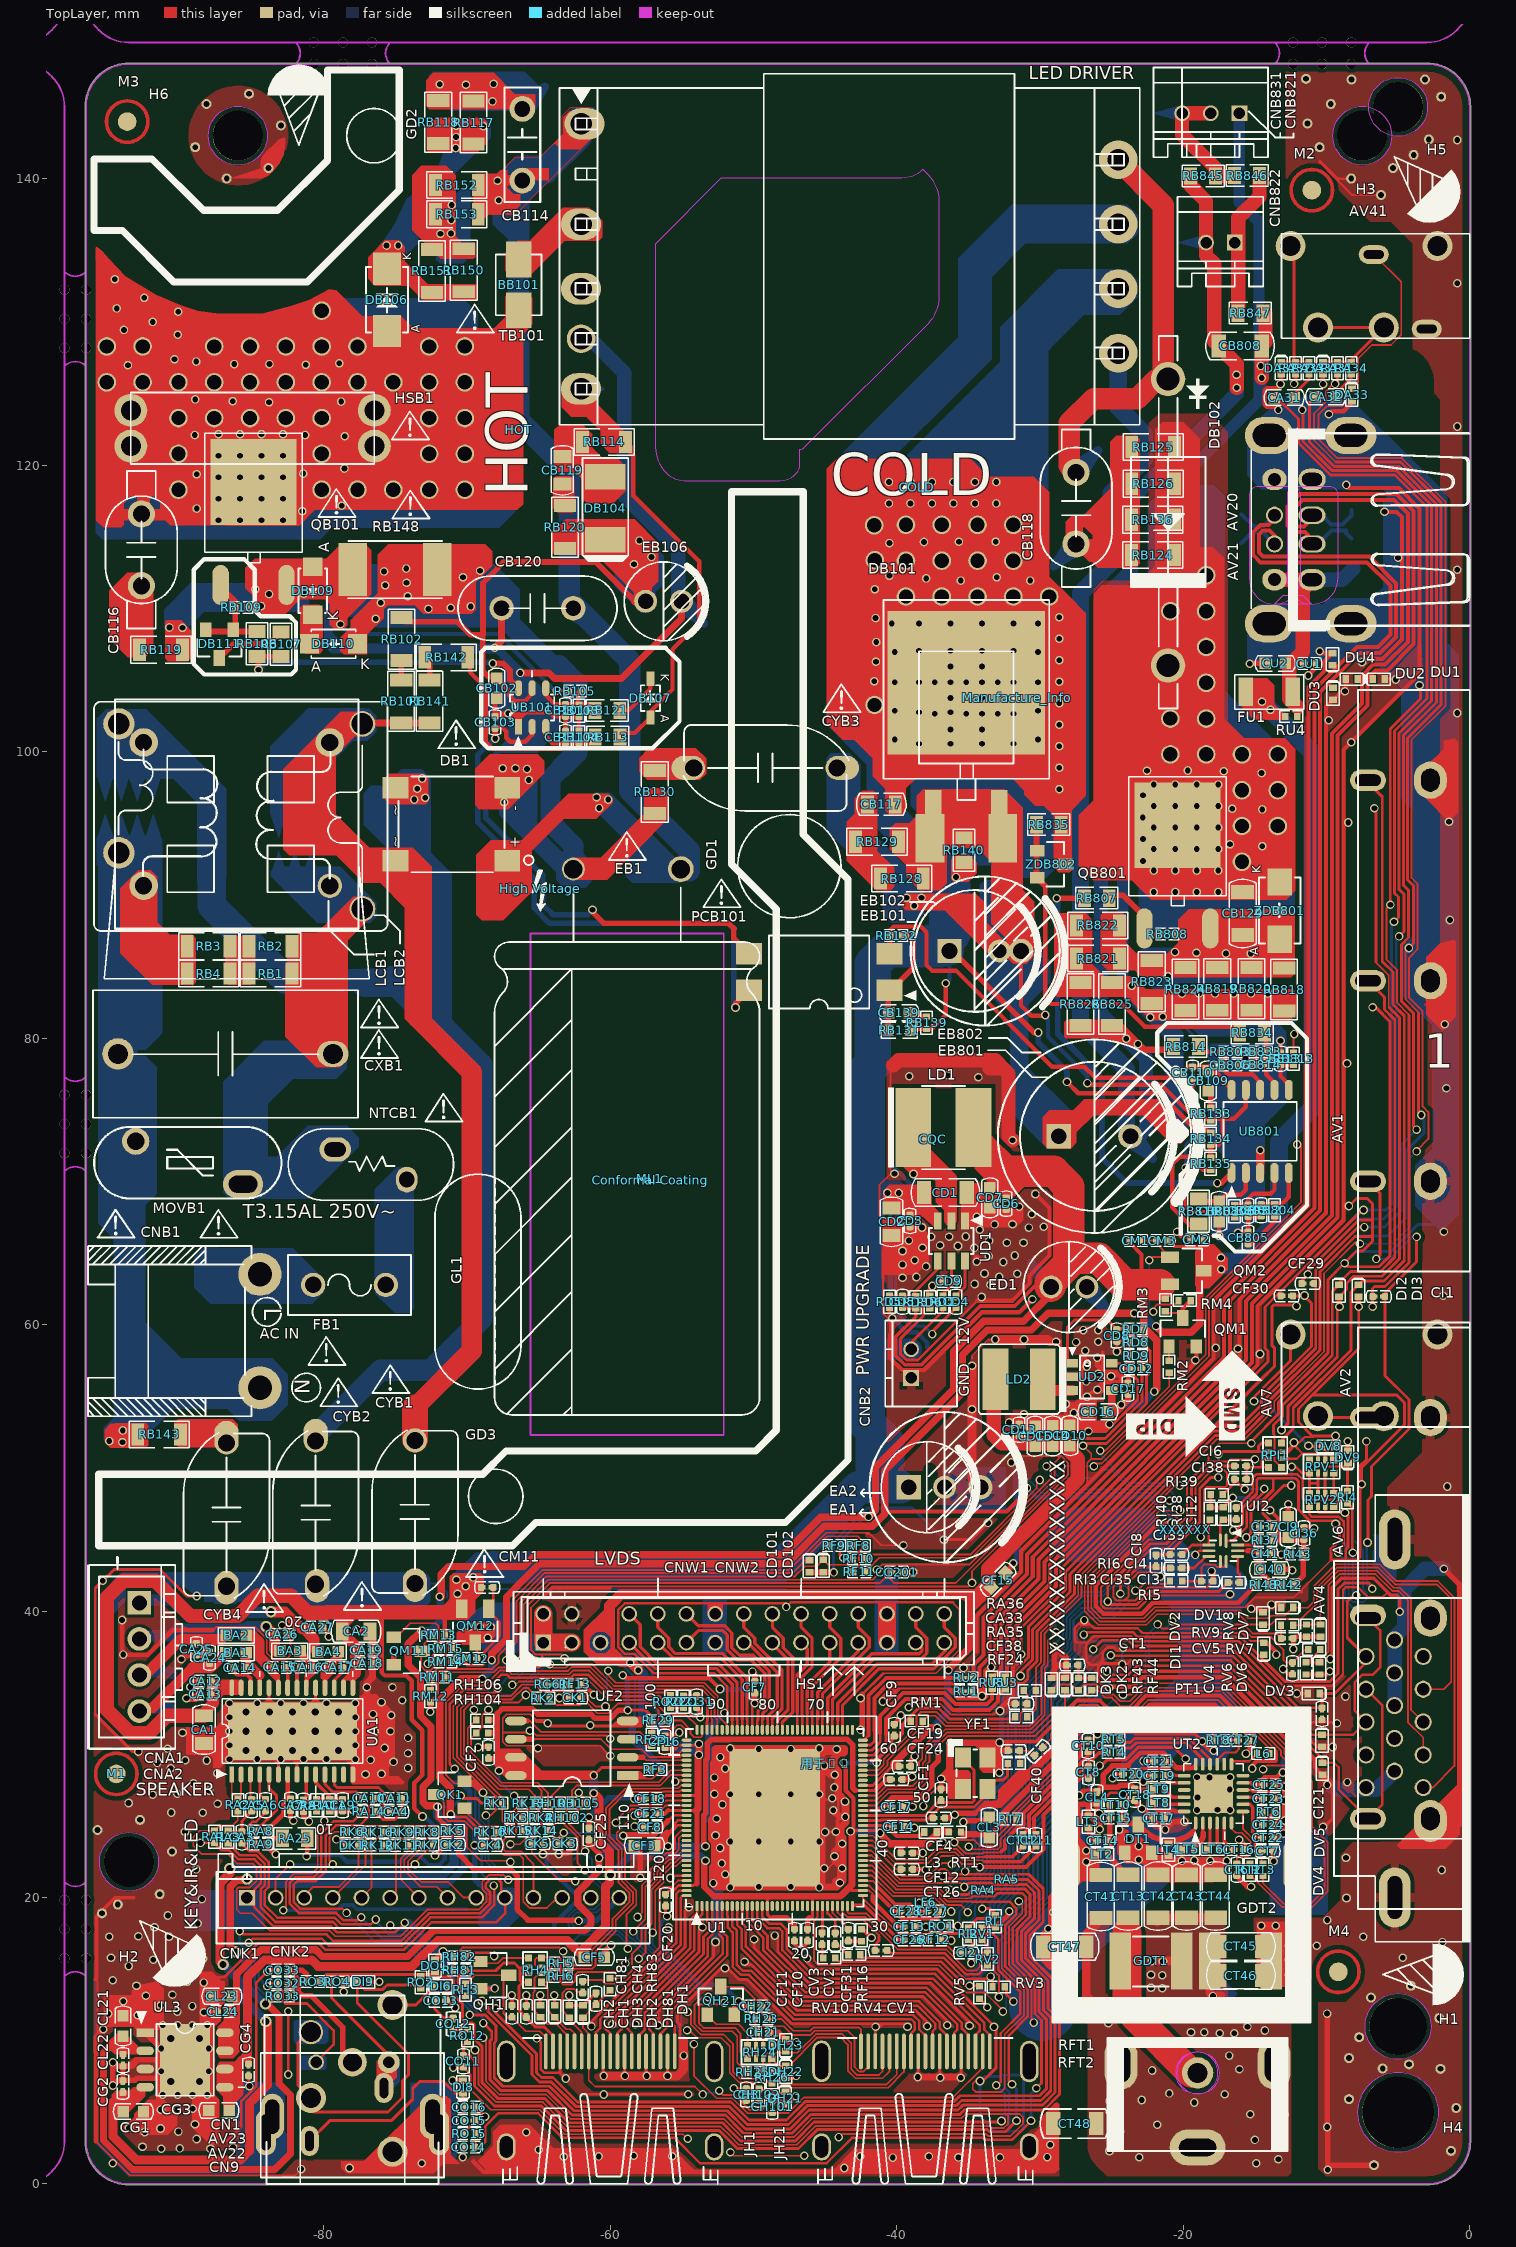
[diagram p0: TopLayer view]
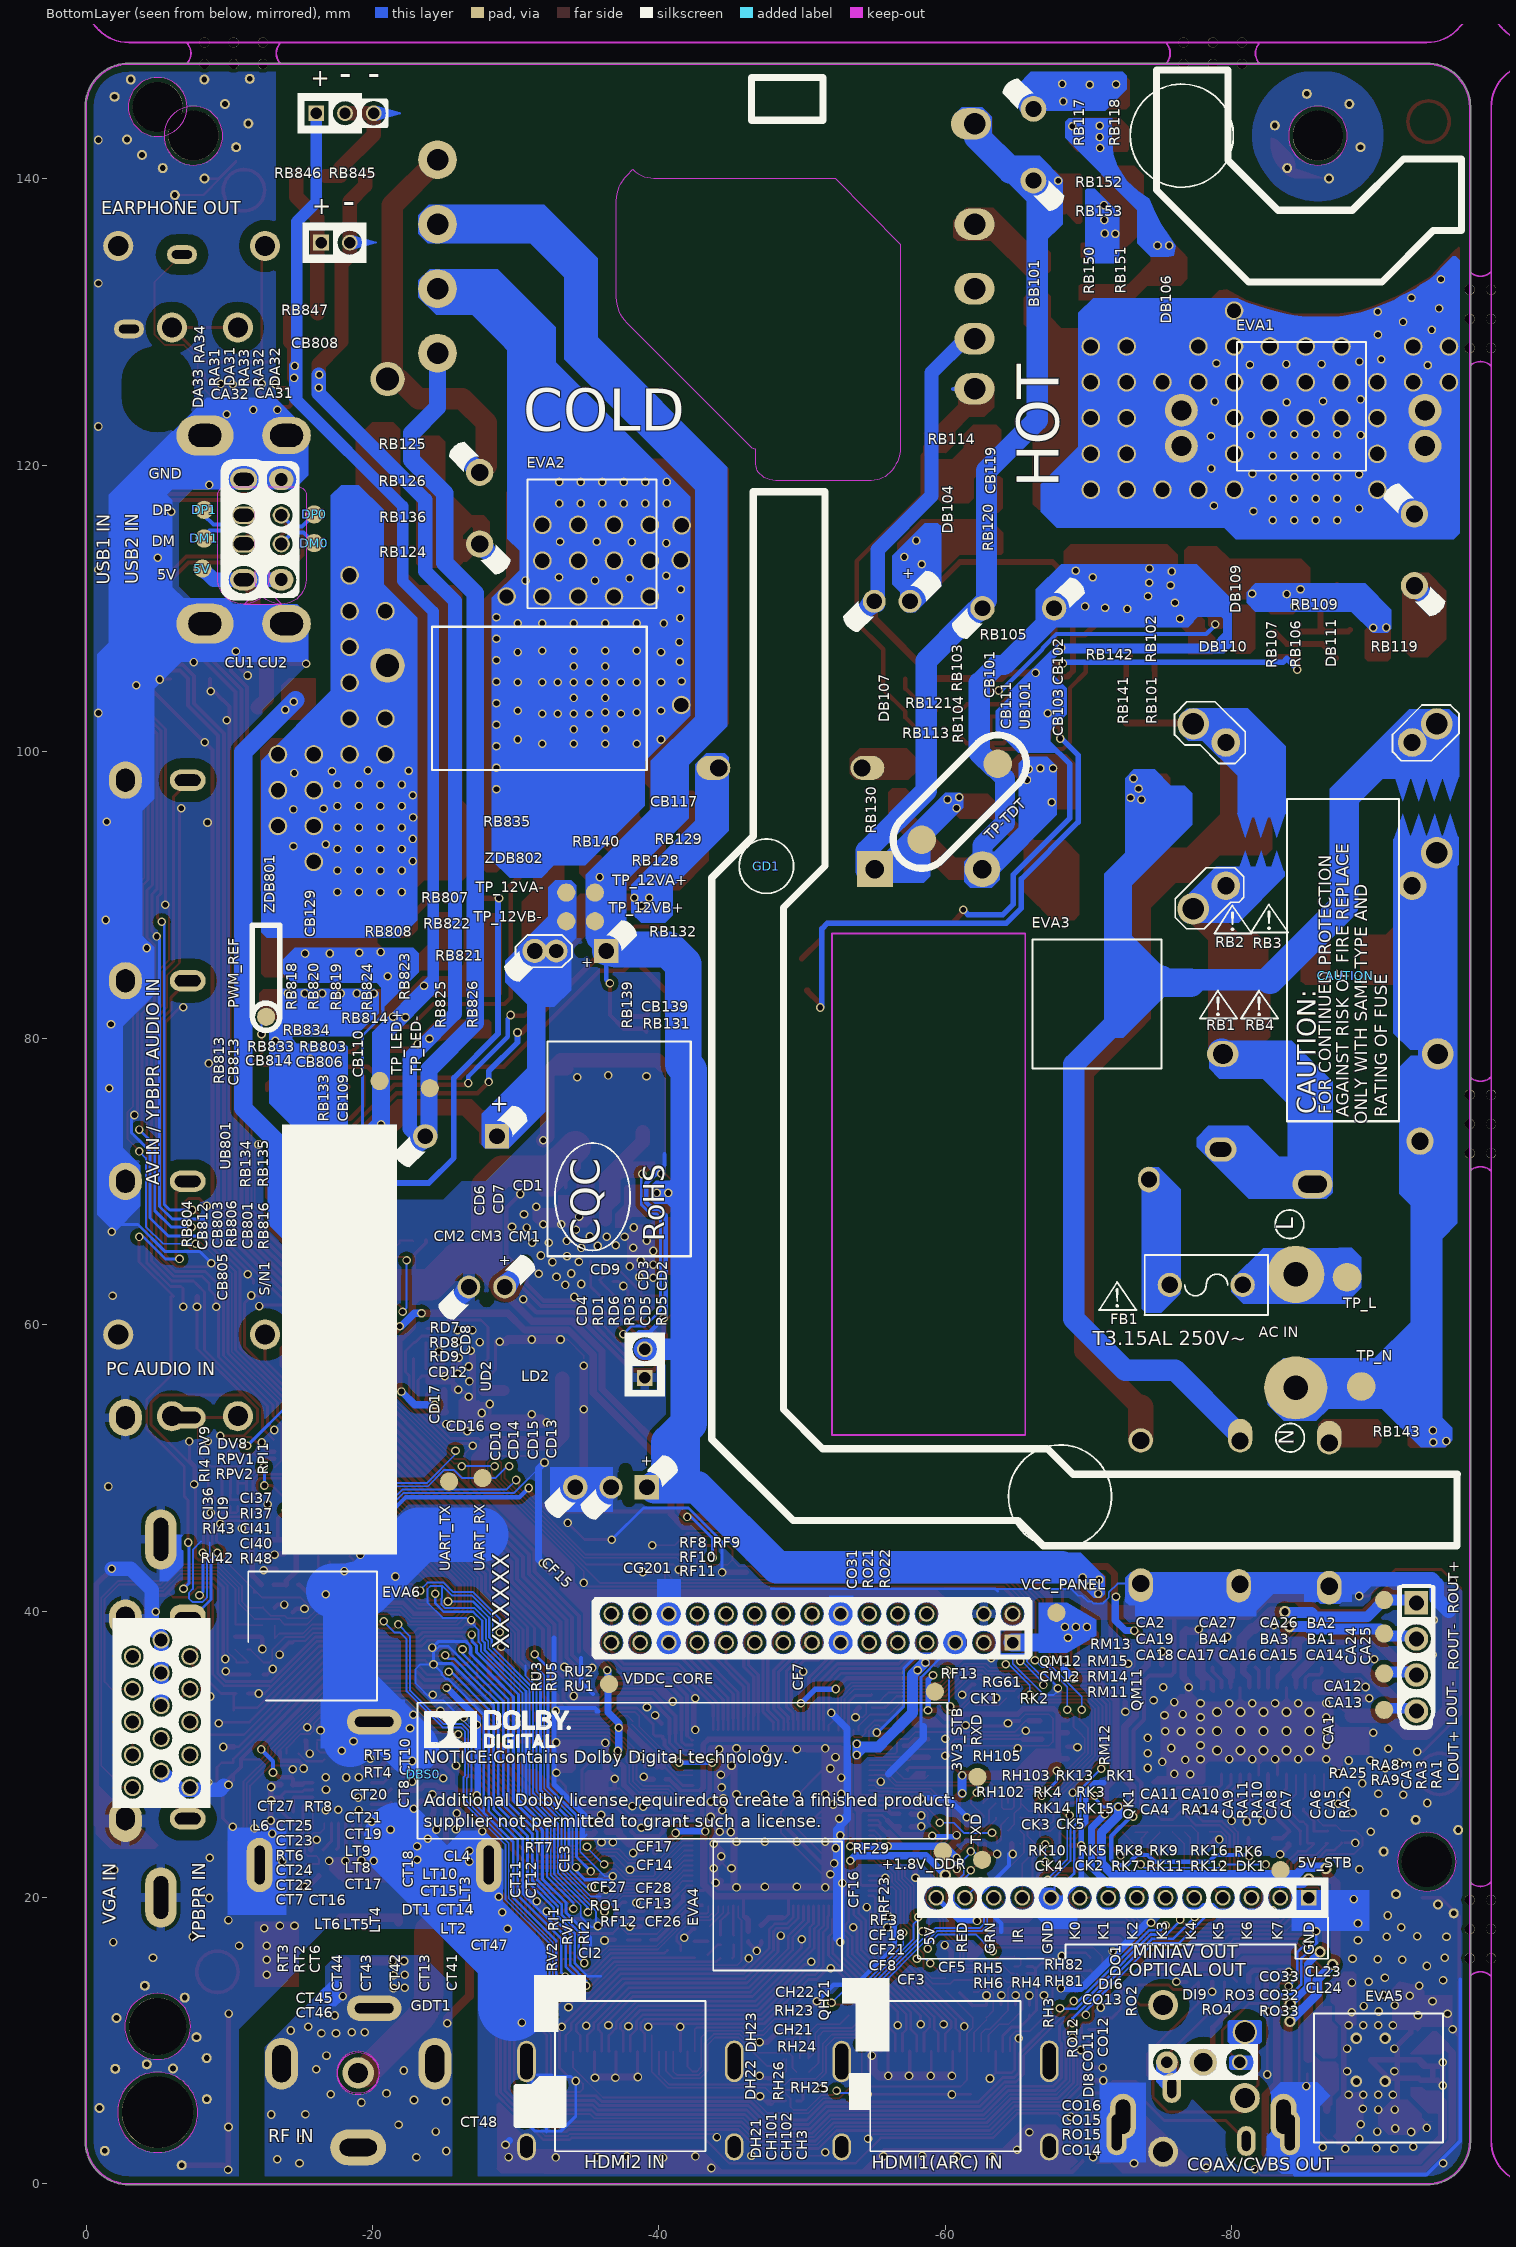
[diagram p1: BottomLayer view, seen from below]
# Altium PCB MISC86372.PcbDoc (part 1 of 16)
Units mm, origin at the board's own origin, x right, y up, seen from the top; angles counter-clockwise.
Board outline 96.73 x 148.13 mm, 2 copper layers (TopLayer, BottomLayer), stack 1.571 mm thick; 578 components, 318 nets, 2702 pads, 836 vias.

## Layer stack, top to bottom
TopLayer: signal copper 0.0356
Dielectric: core 1.5, FR-4, Dk 4.8
BottomLayer: signal copper 0.0356

## Board outline
-96.664,3 -96.664,76.338 -96.664,76.25 ccw(c-96.6,76.25) -96.664,76.249 -96.664,76.25 -96.664,145 cw(c-93.6,145) -93.6,148.064 -3,148.064 cw(c-3,145) 0.064,145 0.064,3 cw(c-3,3) -3,-0.064 -93.6,-0.064 cw(c-93.6,3)

## Design rules (kind name [scope] priority, off if disabled: settings)
Clearance ■KEEPOUT_18mil [(IsTrack Or IsArc) And (AsMM(Width) < 1) And IsKeepOut vs Not IsPad] p1: gap=0.457
Clearance ■HOT_7.2mm [InNetClass('HOT') vs InNetClass('All Nets') And (Not InNetClass('HOT'))] p2: gap=8
Clearance ■DFM_NPTH_10mil [(IsPadHoleValid And (PadIsPlated=false) Or IsPad And ((AsMM(PadXSize_AllLayers) < 1) or (AsMM(PadYSize_AllLayers) < 1 )) And IsKeepout) OR HasFootprintPad('ASSE*','0') vs Not IsPad] p3: gap=0.254
Clearance ■DFM_20mil [(IsTrack or IsArc or IsPad) And IsKeepOut vs IsTrack or IsArc or InPoly] p4: gap=0.508
Clearance ■C_RJ45_2mm [InNetClass('RJ45') vs Not InNetClass('RJ45') AND InNet('*')] p5: gap=2
Clearance ■PWR_A12_8mil [((InNetClass('PWR_A12_8mil') or InNet('*12V*') or InNet('*24V*') or InNet('*PVCC*') or InNet('*19V*') or InNet('*AMP*POWER*') or InNet('*AMP*VCC*') or InNet('*LNB*')) And Not InNetClass('A12_8mil_EXC')) and Not IsPad vs Not InPoly] p6: gap=0.203
Clearance ■PS_L2All_3.2mm [InNet('L-1') vs InNet('*')] p7: gap=3.2
Clearance ■PS_L2LN_1.5mm [InNet('L') Or InNet('L-2') Or InNet('L-3') Or InNet('L-4') Or InNet('L-5') Or InNet('L-6') vs InNet('L-N') And Not(InNet('L') Or InNet('L-2') Or InNet('L-3') Or InNet('L-4') Or InNet('L-5') Or InNet('L-6'))] p8: gap=1.5
Clearance ■PS_N2LN_1.5mm [InNet('N') OR InNet('N-1') OR InNet('N-2') OR InNet('N-3') OR InNet('N-4') OR InNet('N-5') OR InNet('N-6') vs InNet('L-N') And Not (InNet('N') OR InNet('N-1') OR InNet('N-2') OR InNet('N-3') OR InNet('N-4') OR InNet('N-5') OR InNet('N-6'))] p9: gap=1.5
Clearance ■PS_L2LN_3mm [InNet('L') Or InNet('L-2') Or InNet('L-3') Or InNet('L-4') Or InNet('L-5') Or InNet('L-6') vs InNet('*') And Not (InNet('L-N') Or InNet('L') Or InNet('L-2') Or InNet('L-3') Or InNet('L-4') Or InNet('L-5') Or InNet('L-6') Or OnLayer('KeepOutLayer'))] p10: gap=3
Clearance ■PS_N2LN_3mm [InNet('N') OR InNet('N-1') OR InNet('N-2') OR InNet('N-3') OR InNet('N-4') OR InNet('N-5') OR InNet('N-6') vs InNet('*') And Not (InNet('L-N') Or InNet('N') OR InNet('N-1') OR InNet('N-2') OR InNet('N-3') OR InNet('N-4') OR InNet('N-5') OR InNet('N-6') Or OnLayer('KeepOutLayer'))] p11: gap=3
Clearance ■SIP2GND_8mil [HasFootprint('SIP*') vs InPoly] p12: gap=0.203
Clearance ■C_BGA_0P65 [HasFootprint('BGA*0.65*') vs InPoly] p13: gap=0.127
Clearance ■C_BGA_0P8 [HasFootprint('BGA*0.8*') vs InPoly] p14: gap=0.14
Clearance ■Poly_4mil [InPolygonClass('Poly_4mil') vs Not InPoly] p15: gap=0.102
Clearance ■Poly_5mil [InPolygonClass('Poly_5mil') vs Not InPoly] p16: gap=0.127
Clearance ■Poly_6.2mil [InPolygonClass('Poly_6.2mil') vs Not InPoly] p17: gap=0.157
Clearance ■Poly_8mil [InPolygonClass('Poly_8mil') vs Not InPoly] p18: gap=0.203
Clearance ■C_RFGND_1.8mm [InNet('RFGND') vs Not (InNet('RF*IN*') OR InNet('NetCT28*'))] p19: gap=1.8
Clearance ■ESD_10mil [HasFootprint('*IEC*') Or HasFootprint('*-F1*') Or HasFootprint('ANT-RF*')] p20: gap=0.254
Clearance ■ESD_20mil [HasFootprint('*SHIELD*')] p21: gap=0.508
Clearance ■GND_12mil [InNet('GND') vs InPoly] p22: gap=0.305
Clearance ■ESD_30mil [(HasFootprint('SCART*') OR HasFootprint('AV*') OR HasFootprint('DB15*') OR HasFootprint('PHONE*')) vs OnBottomLayer] p23: gap=0.762
Clearance ■ESD_NT_30mil [HasFootprint('SCART*') Or HasFootprint('PHONE-HD-12') Or HasFootprint('PHONE-HD-17') Or HasFootprint('PHONE-HD-10') Or HasFootprint('PHONE-HD-26') vs InNet('GND') And OnTopLayer] p24: gap=0.762
Clearance ■DFM_TH_5mil [HasFootprint('GND') or HasFootprint('TP*') or HasFootprint('MARK*') or HasFootprint('SPARK_GAP') or HasFootprint('USB-HD-3-2') or HasFootprint('PHONE-HS-20') and Not IsRegion vs OnBottomlayer And IsPad OR IsPadHoleValid] p25: gap=0.127
Clearance ■DFM_HS60_5mil [InPadClass('HS60') vs InPadClass('HS60') OR IsPadHoleValid and not InPadClass('VIA5')] p26: gap=0.127
Clearance ■DFM_BCR_4mm [IsPadHoleValid vs IsBoardCutoutRegion] p27: gap=4
Clearance ■DFM_TH_4mm [OnBottomlayer And IsSMTPin vs IsPadHoleValid and not InPadClass('VIA5')] p28: gap=4
Clearance ■DFM_HS60_4mm [InPadClass('HS60') vs IsPad and OnBottomlayer] p29: gap=4
Clearance ■VIA2VIA_6.2mil [(IsVia OR InPadClass('VIA5')) And Not (IsVia And (AsMM(HoleDiameter) = 0.1)) vs (IsVia OR InPadClass('VIA5')) And Not (IsVia And (AsMM(HoleDiameter) = 0.1))] p30: gap=0.157
Clearance ■VIA2VIA_16.2mil [(IsVia OR InPadClass('VIA5')) And Not (IsVia And (AsMM(HoleDiameter) = 0.1)) vs (IsVia OR InPadClass('VIA5')) And Not (IsVia And (AsMM(HoleDiameter) = 0.1))] p31: gap=0.411
Clearance ■VIA2PAD_BGA_5mil [HasFootprint('BGA*') and IsPad vs (IsVia OR InPadClass('VIA5')) And Not (IsVia And (AsMM(HoleDiameter) = 0.1))] p32: gap=0.127
Clearance ■VIA2PAD_6mil [IsVia And Not (IsVia And (AsMM(HoleDiameter) = 0.1)) vs ISPAD and Not HasFootprintPad('*','EPAD') and Not HasFootprintPad('*','257') and Not HasFootprintPad('TP','*') and Not HasFootprintPad('GND','JP*') and Not HasFootprintPad('LQFP216/0.4-2','217') and Not HasFootprintPad('QFP16*','17') and Not HasFootprintPad('QFN16*','17') and Not HasFootprintPad('QFN20*','21') and Not HasFootprintPad('QFN24*','25') and Not HasFootprintPad( 'QFN24*','29') and Not HasFootprintPad('QFN28*','29') and Not HasFootprintPad('QFN32*','33') and Not HasFootprintPad('QFN36*','37') and Not HasFootprintPad('QFN36*','0') and Not HasFootprintPad('QFN32*','0') and Not HasFootprintPad('QFN40*','41') and Not HasFootprintPad('QFN48*','49') and Not HasFootprintPad('LQFP48/0.5-2','49') and Not HasFootprintPad('*SSOP32*','33') and Not HasFootprintPad('SOP8*','9') and Not HasFootprintPad('WSON8/1.27*','9') and Not HasFootprintPad('DFN10/0.5-1*','11') and Not HasFootprintPad('SON16/0.4','9') and Not HasFootprintPad('MSOP10/0.5-1','11') and Not HasFootprintPad('QFN56/0.5','57') and Not HasFootprintPad('LGA31/0.5','3*') and Not InPadClass('VIA_HS60') and Not HasFootprintPad('TSSOP16/0.65-3','17') and Not HasFootprintPad('QFP128/0.5-2','129') and Not HasFootprintPad('QFP128/0.4-5','129') and Not HasFootprintPad('PQFP48*','49') and Not HasFootprintPad('QFP156/0.4-1','157') and Not HasFootprintPad('D2PAK3-TO-252','2') and Not HasFootprintPad('D2PAK3','2')] p33: gap=0.152
Clearance ■PAD2VIA5_6mil [IsPad And ((AsMM(PadXSize_AllLayers) < 2.5) or ((AsMM(PadYSize_AllLayers) < 2.5))) And Not InPadclass('HS60') vs InPadClass('VIA5')] p34: gap=0.152
Clearance "■12mil for Polygon" [InPoly] p35: gap=0.305
Clearance 8mil [All] p36 off: gap=0.203
Clearance 7mil [All] p37 off: gap=0.178
Clearance 6.2mil [All] p38 off: gap=0.157
Clearance 6mil [All] p39 off: gap=0.152
Clearance 5.8mil [All] p40 off: gap=0.147
Clearance 5mil [Not ((IsTrack Or IsArc) And (Layer = 'KeepOutLayer')) vs Not (IsPad or ((IsTrack Or IsArc) And (Layer = 'KeepOutLayer')))] p41 off: gap=0.127
Clearance 4.5mil [Not ((IsTrack Or IsArc) And (Layer = 'KeepOutLayer')) vs Not (IsPad or ((IsTrack Or IsArc) And (Layer = 'KeepOutLayer')))] p42 off: gap=0.114
Clearance "4mil for Minimum" [Not ((IsTrack Or IsArc) And (Layer = 'KeepOutLayer')) vs Not (IsPad or ((IsTrack Or IsArc) And (Layer = 'KeepOutLayer')))] p43: gap=0.102
ComponentClearance ■DFMC_1mm [Not (InComponentClass('Co-Layout') Or HasFootprint('GND')) And (HasFootprint('T/E*') Or HasFootprint('T/PQ*') Or HasFootprint('USB*') Or HasFootprint('HDMI*') Or HasFootprint('USB*') Or HasFootprint('DC-*') Or HasFootprint('AV*') Or HasFootprint('ANT*') Or HasFootprint('PHONE*') Or HasFootprint('CICARD*') Or HasFootprint('CARD*') Or HasFootprint('DVI*') Or HasFootprint('DB*') Or HasFootprint('DP*') Or HasFootprint('DISPLAYPORT*') Or HasFootprint('OPTICAL*') Or HasFootprint('SCART*') Or HasFootprint('RJ45*') Or HasFootprint('USB*') Or HasFootprint('T-*') Or HasFootprint('T/*') Or HasFootprint('200-*') Or HasFootprint('ZhiJia*') Or HasFootprint('Dianpian*') Or HasFootprint('TanPian*') Or HasFootprint('P(*')) vs Not (InComponentClass('Co-Layout') Or HasFootprint('GND'))] p1 off: gap=1 collisioncheckmode=3 verticalgap=1 showdistances=FALSE
ComponentClearance ■DFMC_0.5mm [Not (InComponentClass('Co-Layout') Or HasFootprint('SO-23') Or HasFootprint('DIODE-s0402') Or HasFootprint('GND')) And (HasFootprint('M-*') Or HasFootprint('BGA*') Or HasFootprint('QFP*') Or HasFootprint('QFN*') Or HasFootprint('*DFN*') Or HasFootprint('*SOP*') Or HasFootprint('LGA*') Or HasFootprint('SOIC*') Or HasFootprint('EC*') Or HasFootprint('AC-*') Or HasFootprint('DIODE*') Or HasFootprint('XTAL*') Or HasFootprint('SO-*') Or HasFootprint('L/LC*') Or HasFootprint('L(*') Or HasFootprint('WIFI*') Or HasFootprint('SATA*') Or HasFootprint('POGO*') Or HasFootprint('SOT-223') Or HasFootprint('TO-252') Or HasFootprint('TO-263') Or HasFootprint('KEY*') Or HasFootprint('SW*') Or HasFootprint('DIP*') Or HasFootprint('SIP*') Or HasFootprint('DIP*') Or HasFootprint('CON*') Or HasFootprint('FFC*') Or HasFootprint('FPC*') Or HasFootprint('GDT*') Or HasFootprint('R2512*') Or HasFootprint('R2725*') Or HasFootprint('L2012*') Or HasFootprint('L2520*')) vs Not (InComponentClass('Co-Layout') Or HasFootprint('SO-23') Or HasFootprint('DIODE-s0402') Or HasFootprint('GND'))] p2 off: gap=0.5 collisioncheckmode=3 verticalgap=0.5 showdistances=FALSE
ComponentClearance ■DFMC_0.4mm [Not (InComponentClass('Co-Layout') Or HasFootprint('GND')) And (HasFootprint('C0201*') Or HasFootprint('C0402*') Or HasFootprint('C0603*') Or HasFootprint('C0805*') Or HasFootprint('C1206*') Or HasFootprint('C1210*') Or HasFootprint('R0201*') Or HasFootprint('R0402*') Or HasFootprint('R0603*') Or HasFootprint('R0805*') Or HasFootprint('R*0402*') Or HasFootprint('L0201*') Or HasFootprint('L0402*') Or HasFootprint('L0603*') Or HasFootprint('L0805*') Or HasFootprint('L1206*') Or HasFootprint('DIODE-s0402')) vs Not (InComponentClass('Co-Layout') Or HasFootprint('GND')) And (HasFootprint('C0201*') Or HasFootprint('C0402*') Or HasFootprint('C0603*') Or HasFootprint('C0805*') Or HasFootprint('C1206*') Or HasFootprint('C1210*') Or HasFootprint('R0201*') Or HasFootprint('R0402*') Or HasFootprint('R0603*') Or HasFootprint('R0805*') Or HasFootprint('R*0402*') Or HasFootprint('L0201*') Or HasFootprint('L0402*') Or HasFootprint('L0603*') Or HasFootprint('L0805*') Or HasFootprint('L1206*') Or HasFootprint('DIODE-s0402'))] p3 off: gap=0.4 collisioncheckmode=3 verticalgap=0.4 showdistances=FALSE
ComponentClearance ■DFMC_0.36mm [Not (InComponentClass('Co-Layout') Or HasFootprint('GND')) And HasFootprint('R1206*') vs Not (InComponentClass('Co-Layout') Or HasFootprint('GND')) And HasFootprint('R1206*')] p4 off: gap=0.36 collisioncheckmode=3 verticalgap=0.36 showdistances=FALSE
ComponentClearance ■DFMC_0.25mm [Not (InComponentClass('Co-Layout') Or HasFootprint('GND')) vs Not (InComponentClass('Co-Layout') Or HasFootprint('GND'))] p5 off: gap=0.25 collisioncheckmode=3 verticalgap=0.25 showdistances=FALSE
DiffPairsRouting ■DiffPair_USB_DiffPairsRouting [InDifferentialPairClass('USB')] p1: maxlimit=0.127 minlimit=0.102 mostfreqgap=0.127 maxuncoupledlength=5.08
DiffPairsRouting ■DiffPair_LVDS_DiffPairsRouting [InDifferentialPairClass('LVDS')] p2: maxlimit=0.127 minlimit=0.102 mostfreqgap=0.127 maxuncoupledlength=12.7
DiffPairsRouting ■DiffPair_HDMI_DiffPairsRouting [InDifferentialPairClass('HDMI')] p3: maxlimit=0.127 minlimit=0.102 mostfreqgap=0.127 maxuncoupledlength=5.08
DiffPairsRouting [All] p4: maxlimit=0.254 minlimit=0.254 mostfreqgap=0.254 maxuncoupledlength=12.7
FabricationTestPointUsage TestPointUsage [All] p1: valid=0 allowmultiple=FALSE
FabricationTestpoint Testpoint [All] p1: side=3 testpointundercomponent=TRUE minsize=1.016 maxsize=2.54 preferedsize=1.524 minholesize=0.508 maxholesize=1.016 preferedholesize=0.813 testpointgrid=0.025 allowsidetop=TRUE allowsidebottom=TRUE usegrid=TRUE gridtolerance=0
HoleSize HoleSize_VIA [ISVIA] p1 off: absolutevalues=TRUE maxlimit=0.6 minlimit=0.2 maxpercent=80.000 minpercent=20.000
HoleToHoleClearance Hole2Hole [All] p1 off: gap=0.457 allowstackedmicrovias=FALSE
MatchedLengths DiffPair_USB_MatchedLengths [InDifferentialPairClass('USB')] p1: tolerance=2.54 checknetsindiffpair=TRUE checkdiffpairvsdiffpair=FALSE checkothers=FALSE
MatchedLengths DiffPair_LVDS_MatchedLengths [InDifferentialPairClass('LVDS')] p2: tolerance=2.54 checknetsindiffpair=TRUE checkdiffpairvsdiffpair=FALSE checkothers=FALSE
MatchedLengths DiffPair_HDMI_MatchedLengths [InDifferentialPairClass('HDMI')] p3: tolerance=2.54 checknetsindiffpair=TRUE checkdiffpairvsdiffpair=FALSE checkothers=FALSE
MinimumAnnularRing [All] p1: minimumring=0.1
MinimumSolderMaskSliver ■MiniSolderMaskSliver [All] p1 off: minsoldermaskwidth=0.098
NetAntennae [Not (HasFootprint('ANT-7') or HasFootprint('ANT-BLUECORE'))] p1: netantennaetolerance=1.016
PermittedLayers [All] p1: toplayerpermitted=TRUE bottomlayerpermitted=TRUE
PlaneClearance ■Plane_ESD_30mil [(HasFootprint('SCART*') OR HasFootprint('AV*') OR HasFootprint('DB15*') OR HasFootprint('PHONE*'))] p1: clearance=0.762
PlaneClearance ■Plane_All_9mil [All] p2: clearance=0.229
PlaneConnect ■PlaneOverAll [IsVia or InPadClass('VIA5') Or HasFootprint('ASSE*') OR InPadclass('HS60')] p1: planeconnectstyle=Direct reliefexpansion=0.508 reliefentries=4 reliefconductorwidth=0.254 reliefairgap=0.254
PlaneConnect ■PlaneConnect [All] p2: planeconnectstyle=Relief reliefexpansion=0.305 reliefentries=4 reliefconductorwidth=0.762 reliefairgap=0.305
PolygonConnect ■PourOverAll [IsVia Or InPadclass('HS60') Or InPadClass('VIA5') Or HasFootprint('ASSE*') Or HasFootprint('DIODE-S0402') Or HasFootprint('RCL0524P') Or HasFootprint('SOT-89') OR HasFootprint('SOT-223') OR HasFootprint('TO-252') OR HasFootprint('TO-263') OR HasFootprint('DIODE') OR HasFootprint('SW-HS-2') OR HasFootprint('HDMI*') OR HasFootprint('SO-8B') OR HasFootprint('GND') OR HasFootprint('PHONE*') OR HasFootprint('DIP18/2.54-2') OR HasFootprint('DIP18/2.54-1') OR HasFootprint('UFL-R-SMT-1') OR HasFootprint('WIFI') OR HasFootprint('UM02BS') OR HasFootprint('*SCART*') OR HasFootprint('TSOT23-8/0.65') OR HasFootprint('*SOT-23-*') OR HasFootprint('SOP23-5-1') OR HasFootprint('SOP6/0.95') OR HasFootprint('M-WIFI-2-M603USA1') OR HasFootprint('M-MT7632U') OR HasFootprint('SOP8/1.27') OR HasFootprint('SOP8/1.27-3') vs IsPolygon] p1: connectstyle=Direct reliefconductorwidth=0.254 reliefentries=4 polygonreliefangle="90 Angle"
PolygonConnect ■BGA_0P65 [HasFootprint('BGA*0.65*') vs IsPoly] p2: connectstyle=Relief reliefconductorwidth=0.203 reliefentries=4 polygonreliefangle="45 Angle"
PolygonConnect ■BGA_0P8 [HasFootprint('BGA*0.8*') vs IsPoly] p3: connectstyle=Relief reliefconductorwidth=0.229 reliefentries=4 polygonreliefangle="45 Angle"
PolygonConnect ■Polygon_RFGND [InNet('RFGND')] p4: connectstyle=Direct reliefconductorwidth=0.254 reliefentries=4 polygonreliefangle="90 Angle"
PolygonConnect ■ESD_SCART [HasFootprint('SCART*') vs IsPolygon And onBottomlayer] p5: connectstyle=Direct reliefconductorwidth=0.762 reliefentries=4 polygonreliefangle="90 Angle"
PolygonConnect ■C2Polygon_35mil [HasFootprint('EC*') vs IsPolygon] p6: connectstyle=Relief reliefconductorwidth=0.889 reliefentries=4 polygonreliefangle="90 Angle"
PolygonConnect ■C2Polygon_30mil [(HasFootprint('*0805*') OR HasFootprint('*1206*')) vs IsPolygon] p7: connectstyle=Relief reliefconductorwidth=0.762 reliefentries=4 polygonreliefangle="90 Angle"
PolygonConnect ■C2Polygon_25mil [HasFootprint('*0603*') Or IsThruPin vs IsPolygon] p8: connectstyle=Relief reliefconductorwidth=0.635 reliefentries=4 polygonreliefangle="90 Angle"
PolygonConnect ■C2Polygon_12mil [IsSMTPin vs IsPolygon] p9: connectstyle=Relief reliefconductorwidth=0.305 reliefentries=4 polygonreliefangle="90 Angle"
RoutingVias 0.6_0.4 [All] p1: holewidth=0.4 width=0.6 viastyle="Through Hole" minholewidth=0.4 minwidth=0.6 maxholewidth=0.4 maxwidth=0.6
RoutingVias 0.8_0.5 [All] p2 off: holewidth=0.5 width=0.8 viastyle="Through Hole" minholewidth=0.5 minwidth=0.8 maxholewidth=0.5 maxwidth=0.8
RoutingVias 0.5_0.3 [All] p3 off: holewidth=0.3 width=0.5 viastyle="Through Hole" minholewidth=0.3 minwidth=0.5 maxholewidth=0.3 maxwidth=0.5
RoutingVias 0.45_0.25 [All] p4 off: holewidth=0.25 width=0.45 viastyle="Through Hole" minholewidth=0.25 minwidth=0.45 maxholewidth=0.25 maxwidth=0.45
RoutingVias 0.4_0.2 [All] p5 off: holewidth=0.2 width=0.4 viastyle="Through Hole" minholewidth=0.2 minwidth=0.4 maxholewidth=0.2 maxwidth=0.4
RoutingVias 0.25_0.1 [All] p6 off: holewidth=0.1 width=0.25 viastyle="Through Hole" minholewidth=0.1 minwidth=0.25 maxholewidth=0.1 maxwidth=0.25
SMDNeckDown ■SMDNeckDown_Chip [HasFootprint('FFC*') or HasFootprint('QFP*') or HasFootprint('QFN*') or HasFootprint('HDMI*') or HasFootprint('BGA*')] p1: percent=100.000
SMDToCorner [All] p1 off: distance=40000
ShortCircuit ■ShortCircuit_ViaOnEpad [HasFootprintPad( '*','EPAD') vs IsVia AND InNet('*')] p1: allowed=TRUE
ShortCircuit ■ShortCircuit_JP [HasFootprintPad( 'GND','JP_1K') vs HasFootprintPad( 'GND','JP_2K')] p2: allowed=TRUE
ShortCircuit ■ShortCircuit_0402 [HasFootprintPad('R0402SC','1') OR HasFootprintPad('R0402SC','2') vs HasFootprintPad('R0402SC','3')] p3: allowed=TRUE
ShortCircuit ■ShortCircuit_0603 [HasFootprintPad('R0603SC','1') OR HasFootprintPad('R0603SC','2') vs HasFootprintPad('R0603SC','3')] p4: allowed=TRUE
ShortCircuit ■ShortCircuit_0805 [HasFootprintPad('R0805SC','1') OR HasFootprintPad('R0805SC','2') vs HasFootprintPad('R0805SC','3')] p5: allowed=TRUE
ShortCircuit ■ShortCircuit_1206 [HasFootprintPad('R1206SC','1') OR HasFootprintPad('R1206SC','2') vs HasFootprintPad('R1206SC','3')] p6: allowed=TRUE
ShortCircuit ■ShortCircuit [InNet('*')] p7: allowed=FALSE
SilkToSilkClearance ■Silk2Silk [All] p1: silktosilkclearance=0.127
SilkscreenOverComponentPads ■SilkOverPads [IsText] p1: minsilkscreentomaskgap=0.003
SolderMaskExpansion ■SolderMask_VIA [IsVia] p1: expansion=0.13
SolderMaskExpansion ■SolderMask_All [All] p2: expansion=0.051
UnRoutedNet ■UnRoutedNet [All] p1:
ViasUnderSMD [All] p1: allowed=FALSE
Width ■Width_2.5mm [InFromToClass('Width_2.5mm')] p1: maxlimit=2.5 minlimit=2.5 preferedwidth=2.5
Width ■Width_1.5mm [InFromToClass('Width_1.5mm')] p2: maxlimit=1.5 minlimit=1.5 preferedwidth=1.5
Width ■DiffPair_USB_Width [InDifferentialPairClass('USB')] p3: maxlimit=0.279 minlimit=0.102 preferedwidth=0.279
Width ■DiffPair_LVDS_Width [InDifferentialPairClass('LVDS')] p4: maxlimit=0.178 minlimit=0.102 preferedwidth=0.178
Width ■DiffPair_HDMI_Width [InDifferentialPairClass('HDMI')] p5: maxlimit=0.178 minlimit=0.102 preferedwidth=0.178
Width [All] p6: maxlimit=12.7 minlimit=0.076 preferedwidth=0.203
14 further rules are at their usual default settings.

## Classes and differential pairs
net class POWER: 12V 12V_OVP BRO D_QB101 D_QB801 FB GND L L-1 L-2 L-3 L-N LED_FB N-1 N-2 N-3 NetBB101_2 NetCB101_1 NetCB102_1 NetCB103_1 NetCB109_2 NetCB114_2 NetCB116_2 NetCB117_2 NetCB118_2 NetCB119_1 NetCB119_2 NetCB139_1 NetCB139_2 NetCB801_1 NetCB803_1 NetCB805_2 NetCB806_1 NetCB812_2 NetCB813_2 NetCB814_1 NetCNB821_2 NetCNB822_1 NetCYB3_1 NetDB107_K NetDB109_A NetDB109_K NetDB111_1 NetDB111_2 NetQB801_G NetRB106_1 NetRB834_2 NetTB101_2 NetTB101_4 PWM_REF SGND SNB-D SNB-RM SYN VBL-COIL Vbridge VBRO VCOMP VGS1 VREF VSTB
net class HOT: 12V_OVP BRO D_QB101 L L-1 L-2 L-3 L-N N-1 N-2 N-3 NetBB101_2 NetCB101_1 NetCB102_1 NetCB103_1 NetCB114_2 NetCB116_2 NetCB119_1 NetCB119_2 NetCYB3_1 NetDB107_K NetDB109_A NetDB109_K NetDB111_1 NetDB111_2 NetRB106_1 SGND SNB-D SNB-RM Vbridge VBRO VSTB
component class TV#09_Tuner: CL3 CL4 CT1 CT6 CT7 CT8 CT9 CT10 CT11 CT12 CT13 CT14 CT15 CT16 CT17 CT18 CT19 CT20 CT21 CT22 CT23 CT24 CT25 CT26 CT27 CT41 CT42 CT43 CT44 CT45 CT46 CT47 CT48 DT1 GDT1 GDT2 LT2 LT3 LT4 LT5 LT6 LT8 LT9 LT10 PT1 RFT1 RFT2 RT1 RT2 RT3 RT4 RT5 RT6 RT7 RT8 UT2
component class TV#08_AMP: AV41 BA1 BA2 BA3 BA4 CA1 CA2 CA3 CA4 CA5 CA6 CA7 CA8 CA9 CA10 CA11 CA12 CA13 CA14 CA15 CA16 CA17 CA18 CA19 CA24 CA25 CA26 CA27 CA31 CA32 CA33 CNA1 CNA2 DA31 DA32 DA33 EA1 EA2 LOUT+ LOUT- RA1 RA2 RA3 RA4 RA5 RA8 RA9 RA10 RA11 RA14 RA25 RA31 RA32 RA33 RA34 RA35 RA36 ROUT+ ROUT- UA1
component class TV#07_HDMI: CD101 CD102 CH1 CH2 CH3 CH4 CH21 CH22 CH81 CH101 CH102 DH1 DH2 DH3 DH21 DH22 DH23 DH81 JH1 JH21 QH1 QH21 RH3 RH4 RH5 RH6 RH23 RH24 RH25 RH26 RH81 RH82 RH83 RH102 RH103 RH104 RH105 RH106 RXD TXD
component class TV#06_COAX&MINIAV&OPTICAL&USB: 5V AV20 AV21 AV22 AV23 CN1 CN9 CO11 CO12 CO13 CO14 CO15 CO16 CO31 CO32 CO33 CU1 CU2 DI6 DI8 DI9 DM0 DM1 DO1 DP0 DP1 DU1 DU2 DU3 DU4 FU1 RO1 RO2 RO3 RO4 RO12 RO15 RO21 RO22 RO33 RU1 RU2 RU3 RU4 RU5
component class TV#05_AV&YPBPR&VGA: AV1 AV2 AV4 AV6 AV7 CI1 CI2 CI3 CI4 CI5 CI6 CI7 CI8 CI9 CI12 CI21 CI35 CI36 CI37 CI38 CI39 CI40 CI41 CV1 CV2 CV3 CV4 CV5 DI1 DI2 DI3 DV1 DV2 DV3 DV4 DV5 DV6 DV7 DV8 DV9 RF8 RF9 RF10 RF11 RI1 RI2 RI3 RI4 RI5 RI6 RI37 RI38 RI39 RI40 RI42 RI43 RI48 RPI1 RPV1 RPV2 RV1 RV2 RV3 RV4 RV5 RV6 RV7 RV8 RV9 RV10 UART_RX UART_TX UI2
component class TV#04_LVDS: CM11 CM12 CNW1 CNW2 QM11 QM12 RM11 RM12 RM13 RM14 RM15 VCC_PANEL
component class TV#03_IR&KEY: CK1 CK2 CK3 CK4 CK5 CNK1 CNK2 DK1 QK1 RK1 RK2 RK3 RK4 RK5 RK6 RK7 RK8 RK9 RK10 RK11 RK12 RK13 RK14 RK15 RK16
component class TV#02_MS3553V53&U63&3663LWA: CF1 CF2 CF3 CF4 CF5 CF7 CF8 CF9 CF10 CF11 CF12 CF13 CF14 CF15 CF16 CF17 CF18 CF19 CF20 CF21 CF24 CF25 CF26 CF27 CF28 CF29 CF30 CF31 CF38 CF40 CG201 DK2 DK3 L3 L6 LF6 RF3 RF12 RF13 RF16 RF23 RF24 RF29 RF43 RF44 RG61 U1 UF2 YF1
component class TV#01_POWER: 3V3_STB 5V_STB +1.8V_DDR CD1 CD2 CD3 CD4 CD5 CD6 CD7 CD8 CD9 CD10 CD12 CD13 CD14 CD15 CD16 CD17 CG1 CG2 CG3 CG4 CL21 CL22 CL23 CL24 CM1 CM2 CM3 ED1 LD1 LD2 QM1 QM2 RD1 RD3 RD5 RD6 RD7 RD8 RD9 RM1 RM2 RM3 RM4 UD1 UD2 UL3 VDDC_CORE
component class SCH_info: DBS0 HS1 XXXXXX XXXXXXXXXXXXXX 用于U1
component class PS#01_XXXXXXXXXXXXXX: BB101 CB101 CB102 CB103 CB109 CB110 CB111 CB114 CB116 CB117 CB118 CB119 CB120 CB129 CB139 CB801 CB803 CB805 CB806 CB808 CB812 CB813 CB814 CNB1 CNB2 CNB821 CNB822 CNB831 CNB832 "Conformal Coating" CXB1 CYB1 CYB2 CYB3 CYB4 DB1 DB101 DB102 DB104 DB106 DB107 DB109 DB110 DB111 EB1 EB101 EB102 EB106 EB801 EB802 EVA1 EVA2 EVA3 EVA4 EVA5 EVA6 FB1 GD1 GD2 GD3 GL1 HSB1 HSB2 HSB3 HSB4 LCB1 LCB2 ML1 MOVB1 NTCB1 PCB101 PWM_REF QB101 QB801 RB1 RB2 RB3 RB4 RB101 RB102 RB103 RB104 RB105 RB106 RB107 RB109 RB113 RB114 RB117 RB118 RB119 RB120 RB121 RB124 RB125 RB126 RB128 RB129 RB130 RB131 RB132 RB133 RB134 RB135 RB136 RB139 RB140 RB141 RB142 RB143 RB148 RB150 RB151 RB152 RB153 RB803 RB804 RB806 RB807 RB808 RB813 RB814 RB816 RB818 RB819 RB820 RB821 RB822 RB823 RB824 RB825 RB826 RB833 RB834 RB835 RB845 RB846 RB847 TB101 TP-TDT TP_12VA+ TP_12VA- TP_12VB+ TP_12VB- TP_L TP_LED+ TP_LED- TP_N UB101 UB801 ZDB801 ZDB802
component class PCB_info: AI_V CAUTION COLD CQC H1 H2 H3 H4 H5 H6 "High Voltage" HOT M1 M2 M3 M4 Manufacture_Info S/N1
polygon class Poly_5mil: 5
pad class VIA5: Free-via5
polygon class Poly_6.2mil: 6.2

## Components (designator, comment, footprint, x,y, rotation, side; value= is the part's Value field where it differs from the comment)
3V3_STB "TEST" TP -59.258,34.366 r270 bottom
5V "DM0" TP -8.128,112.776 r180 bottom
5V_STB "TEST" TP -83.388,21.908 r90 bottom
+1.8V_DDR "TEST" TP -59.817,23.216 r90 bottom
AI_V "AI_GRIPPER_V" AI_GRIPPER_V 30.243,27.653 r90 top
AV1 "RCA jack,RCA Jack,AV3,H,Yellow、White、Red,CH5.5,D14,Seal,DIP,AV3-8.4-15C,JSL(MI material)" AV3-H14-15#1 0,84 r90 top locked
AV2 "NC/RCA jack,RCA Jack,AV3,H,Yellow、White、Red,CH5.5,D14,Seal,DIP,AV3-8.4-15C,JSL(MI material)" AV3-H14-15#2 0,39.5 r90 top
AV4 "RCA jack,RCA Jack,AV3,H,Green、Blue、Red,CH5.5,D14,Seal,DIP,AV3-8.4-15C,JSL" AV3-H14-15#3 0,39.5 r90 top locked
AV6 "NC/WLHD-051A" DB15-HF-1 0,32.5 r90 top locked
AV7 "NC/Earphone jack,Earphone Jack,H,Φ3.5,CH7.0,Black,Seal,DIP,PJ-373,JSL" PHONE-HD-41 0,56.5 r90 top locked
AV20 "USB jack,USB Jack,H,Single,flange,DIP,WLUS-050F USB,WLCO" USB1-HD-2 1.947,115.5 r90 top locked
AV21 "NC/USB jack,USB Jack,H,Double,Black,flange,DIP,WLUS-074B,WLCO" USB2-HD-1 2,115.5 r90 top locked
AV22 "RCA jack,RCA Jack,AV1,H,Orange,CH5.5,Seal,DIP,RCA-143A-EP-07,CS" AV1-H-4 -78,0.45 r0 top locked
AV23 "NC/Optical jack,OPTICAL,H,DIP,182500191,VAST" OPTICAL-HD-3 -78,0 r0 top locked
AV41 "Earphone jack,Earphone Jack,H,Φ3.5,CH7.0,Black,switch,Seal,DIP,PJ-373A,JSL" PHONE-HD-42#1 0,132.5 r90 top locked
BA1 "Ferrite bead,BEAD,600ohm,0603,2A,SMD,TP,EPZ1608E601-2R0TF,Sunlord" L0603 -86.12,37.073 r180 top
BA2 "Ferrite bead,BEAD,600ohm,0603,2A,SMD,TP,EPZ1608E601-2R0TF,Sunlord" L0603 -86.114,38.295 r180 top
BA3 "Ferrite bead,BEAD,600ohm,0603,2A,SMD,TP,EPZ1608E601-2R0TF,Sunlord" L0603 -82.372,37.211 r180 top
BA4 "Ferrite bead,BEAD,600ohm,0603,2A,SMD,TP,EPZ1608E601-2R0TF,Sunlord" L0603 -79.705,37.16 r180 top